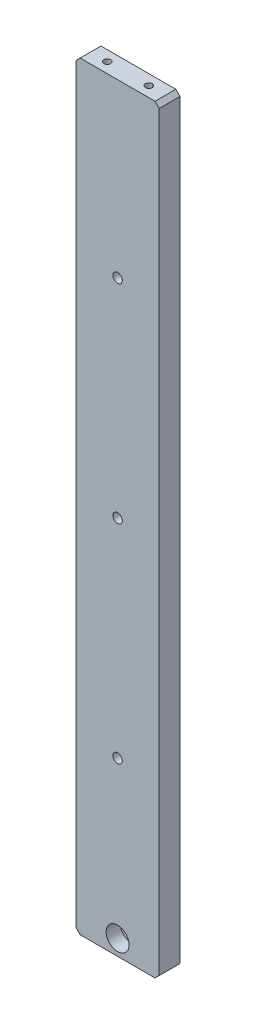
SolidWorks part; units mm, degrees
material "A6061-T6"
ref_plane "Front Plane" through (0, 0, 0) normal (0, 0, 1) x (1, 0, 0)
ref_plane "Top Plane" through (0, 0, 0) normal (0, 1, 0) x (1, 0, 0)
ref_plane "Right Plane" through (0, 0, 0) normal (1, 0, 0) x (0, 0, -1)
sketch "Sketch1" plane through (0, 0, 0) normal (0, 0, 1) x (1, 0, 0)
  line L1 (20, -182.5) -> (-20, -182.5)
  line L2 (20, -182.5) -> (20, 182.5)
  line L3 (20, 182.5) -> (-20, 182.5)
  line L4 (-20, -182.5) -> (-20, 182.5)
  line L5 (20, -182.5) -> (-20, 182.5) construction
  line L6 (20, 182.5) -> (-20, -182.5) construction
  point P0 (0, 0)
  dimension "D1" = 365
  dimension "D2" = 40
extrude "Boss-Extrude1" add sketch "Sketch1" along normal mid plane 10
hole_wizard "M4 Tapped Hole2" positions "Sketch10" profile "Sketch9" tap size "M4" standard "GB"
sketch "Sketch10" plane through (0, 182.5, 0) normal (0, 1, 0) x (1, 0, 0)
  line L0 (0, 12.5017) -> (0, 0) construction
  line L1 (0, 0) -> (-34.6915, 0) construction
  line L3 (-20, -5) -> (-20, 5) construction
  point P9 (-10, 0)
  point P20 (10, 0)
  dimension "D1" = 10
sketch "Sketch9" plane through (10, 182.5, 0) normal (1, 0, 0) x (0, 0, 1)
  line L0 (0, 0) -> (0, 11.0914)
  line L1 (0, 11.0914) -> (1.65, 10.1)
  line L2 (1.65, 10.1) -> (1.65, 0)
  line L5 (1.65, 0) -> (0, 0)
  line L10 (0, 11.0914) -> (-1.65, 10.1) construction
  line L11 (0, -6.35) -> (0, 107.95) construction
  dimension "螺纹孔钻头直径" = 3.3
  dimension "螺纹孔钻头深度" = 10.1
  dimension "导头角度" = 118
cosmetic thread "Hole thread 7" parameters "D1"=8, "D2"=4
cosmetic thread "Hole thread 8" parameters "D1"=8, "D2"=4
hole_wizard "Hex socket cap screw hole type 1" positions "Sketch13" profile "Sketch14" counterbore size "M6" standard "GB" end condition through all
sketch "Sketch13" plane through (0, 0, 5) normal (0, 0, 1) x (1, 0, 0)
  line L0 (-20, -182.5) -> (20, -182.5) construction
  line L2 (0, -182.5) -> (0, -175) construction
  point P0 (0, -175)
  dimension "D1" = 7.5
sketch "Sketch14" plane through (0, -175, 5) normal (1, 0, 0) x (0, -1, 0)
  line L0 (0, 0) -> (0, 10)
  line L1 (0, 10) -> (3.3, 10)
  line L3 (3.3, 10) -> (3.3, 6.8)
  line L4 (3.3, 6.8) -> (5.5, 6.8)
  line L5 (5.5, 6.8) -> (5.5, 0)
  line L7 (5.5, 0) -> (0, 0)
  line L11 (0, -6.35) -> (0, 107.95) construction
  dimension "通孔孔直径" = 6.6
  dimension "通孔孔深度" = 10
  dimension "柱形沉头孔直径" = 11
  dimension "柱形沉头孔深度" = 6.8
hole_wizard "M5 Tapped Hole1" positions "Sketch21" profile "Sketch22" tap size "M5" standard "GB"
sketch "Sketch21" plane through (-20, 0, 0) normal (-1, 0, 0) x (0, 0, 1)
  line L1 (0, 100) -> (0, -100) construction
  point P18 (0, 0)
  point P21 (0, 100)
  point P23 (0, -100)
  dimension "D1" = 200
sketch "Sketch22" plane through (-20, 0, 0) normal (0, 1, 0) x (0, 0, 1)
  line L0 (0, 0) -> (0, 15.2618)
  line L1 (0, 15.2618) -> (2.1, 14)
  line L2 (2.1, 14) -> (2.1, 0)
  line L5 (2.1, 0) -> (0, 0)
  line L10 (0, 15.2618) -> (-2.1, 14) construction
  line L11 (0, -6.35) -> (0, 107.95) construction
  dimension "螺纹孔钻头直径" = 4.2
  dimension "螺纹孔钻头深度" = 14
  dimension "导头角度" = 118
cosmetic thread "Hole thread 17" parameters "D1"=10, "D2"=5
cosmetic thread "Hole thread 18" parameters "D1"=10, "D2"=5
cosmetic thread "Hole thread 19" parameters "D1"=10, "D2"=5
chamfer "Chamfer1" distance 2 angle 45 4 edges at (-20, -182.5, 0) (20, -182.5, 0) (-20, 182.5, 0) (20, 182.5, 0)
hole_wizard "Hex socket cap screw hole type 2" positions "Sketch23" profile "Sketch24" counterbore size "M4" standard "GB" end condition through all
sketch "Sketch23" plane through (0, 0, -5) normal (0, 0, -1) x (-1, 0, 0)
  line L3 (0, -100) -> (0, 100) construction
  point P0 (0, 100)
  point P10 (0, 0)
  point P12 (0, -100)
  dimension "D1" = 200
sketch "Sketch24" plane through (0, 100, -5) normal (1, 0, 0) x (0, 1, 0)
  line L0 (0, 0) -> (0, 10)
  line L1 (0, 10) -> (2.25, 10)
  line L3 (2.25, 10) -> (2.25, 4.6)
  line L4 (2.25, 4.6) -> (4, 4.6)
  line L5 (4, 4.6) -> (4, 0)
  line L7 (4, 0) -> (0, 0)
  line L11 (0, -6.35) -> (0, 107.95) construction
  dimension "通孔孔直径" = 4.5
  dimension "通孔孔深度" = 10
  dimension "柱形沉头孔直径" = 8
  dimension "柱形沉头孔深度" = 4.6
